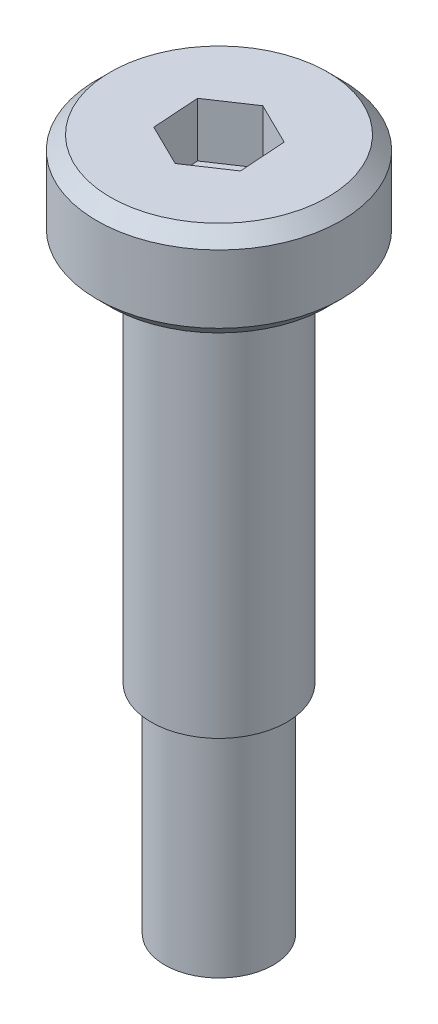
SolidWorks part; units mm, degrees
ref_plane "Front Plane" through (0, 0, 0) normal (0, 0, 1) x (1, 0, 0)
ref_plane "Top Plane" through (0, 0, 0) normal (0, 1, 0) x (1, 0, 0)
ref_plane "Right Plane" through (0, 0, 0) normal (1, 0, 0) x (0, 0, -1)
sketch "Sketch1" plane through (0, 0, 0) normal (0, 0, 1) x (1, 0, 0)
  line L0 (0, 0) -> (0, 25.5)
  line L1 (0, 25.5) -> (-4.5, 25.5)
  line L2 (-4.5, 25.5) -> (-4.5, 22)
  line L3 (-4.5, 22) -> (-2.5, 22)
  line L4 (-2.5, 22) -> (-2.5, 8)
  line L5 (-2.5, 8) -> (-2, 8)
  line L6 (-2, 8) -> (-2, 0)
  line L7 (-2, 0) -> (0, 0)
  dimension "D1" = 2
  dimension "D2" = 8
  dimension "D3" = 2.5
  dimension "D4" = 14
  dimension "D5" = 4.5
  dimension "D6" = 3.5
revolve "Revolve1" add sketch "Sketch1" angle 360 about L0
sketch "Sketch2" plane through (0, 25.5, 0) normal (0, 1, 0) x (1, 0, 0)
  line L1 (1.5541, -0.7647) -> (1.4393, 0.9635)
  line L2 (1.4393, 0.9635) -> (-0.1148, 1.7282)
  line L3 (-0.1148, 1.7282) -> (-1.5541, 0.7647)
  line L4 (-1.5541, 0.7647) -> (-1.4393, -0.9635)
  line L5 (-1.4393, -0.9635) -> (0.1148, -1.7282)
  line L6 (0.1148, -1.7282) -> (1.5541, -0.7647)
  circle A0 centre (0, 0) radius 1.5 construction
  dimension "D1" = 3
extrude "Cut-Extrude1" cut sketch "Sketch2" against normal blind 2
chamfer "Chamfer1" distance 0.5 angle 45 2 edges at (4.5, 25.5, 0) (4.5, 22, 0)
